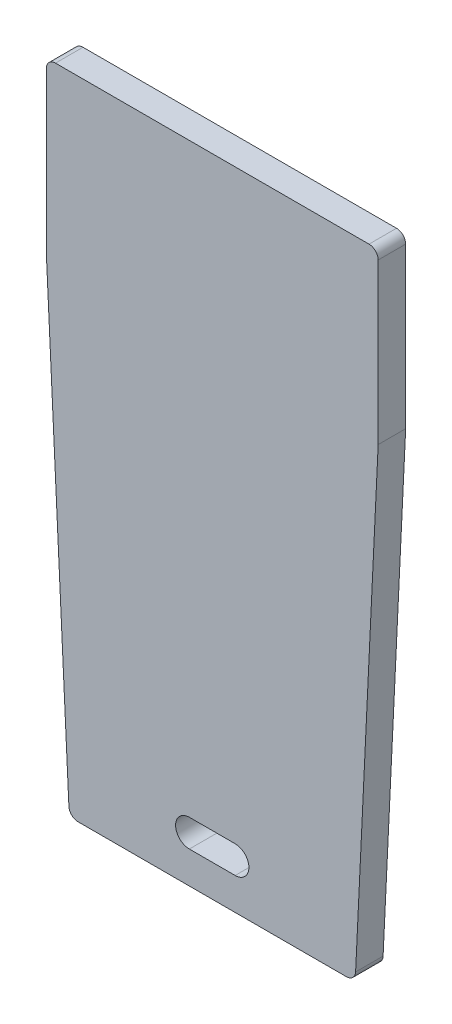
from build123d import *

# Parameters (mm, degrees)
BOSS_EXTRUDE1_DEPTH = 9.525


with BuildPart() as part:
    # Sketch1 → Boss-Extrude1 (new, symmetric)
    with BuildSketch(Plane.XY):
        with BuildLine():
            Line((108.65, 415.8), (-108.65, 415.8))
            ThreePointArc((-108.65, 415.8), (-113.140128061, 413.940128061), (-115, 409.45))
            Line((-115, 409.45), (-115, 298.68))
            Line((-115, 298.68), (-99.351565081, -25.705969286))
            ThreePointArc((-99.351565081, -25.705969286), (-97.389556909, -29.997031921), (-93.008940798, -31.75))
            Line((-93.008940798, -31.75), (93.008940798, -31.75))
            ThreePointArc((93.008940798, -31.75), (97.389556909, -29.997031921), (99.351565081, -25.705969286))
            Line((99.351565081, -25.705969286), (115, 298.68))
            Line((115, 298.68), (115, 409.45))
            ThreePointArc((115, 409.45), (113.140128061, 413.940128061), (108.65, 415.8))
        make_face()
        with BuildLine():
            Line((-15.875, 9.525), (15.875, 9.525))
            ThreePointArc((15.875, 9.525), (25.4, 0), (15.875, -9.525))
            Line((15.875, -9.525), (-15.875, -9.525))
            ThreePointArc((-15.875, -9.525), (-25.4, 0), (-15.875, 9.525))
        make_face(mode=Mode.SUBTRACT)
    extrude(amount=BOSS_EXTRUDE1_DEPTH, both=True)


solid = part.part
